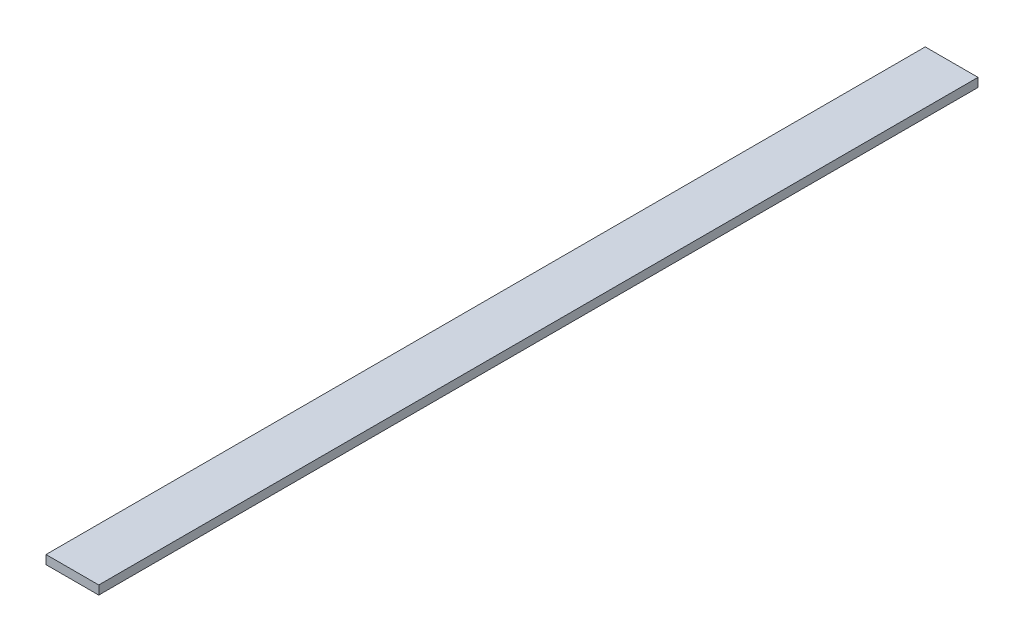
from build123d import *

# Parameters (mm, degrees)
SKETCH_1_W      = 18
SKETCH_1_H      = 3
EXTRUDE_1_DEPTH = 300


with BuildPart() as part:
    # 草图1 → 凸台-拉伸1 (new body)
    with BuildSketch(Plane.XY):
        Rectangle(SKETCH_1_W, SKETCH_1_H)
    extrude(amount=EXTRUDE_1_DEPTH)


solid = part.part
